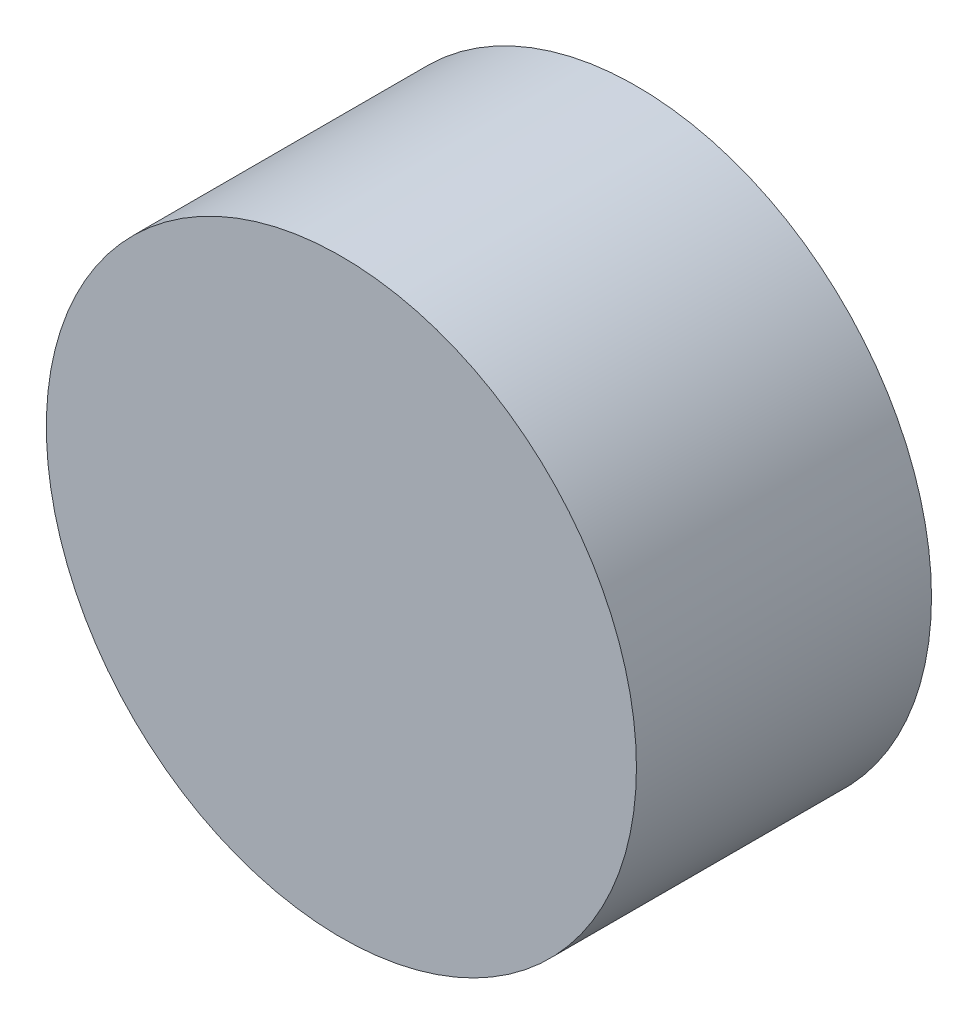
SolidWorks part; units mm, degrees
material "普通碳钢"
ref_plane "Front Plane" through (0, 0, 0) normal (0, 0, 1) x (1, 0, 0)
ref_plane "Top Plane" through (0, 0, 0) normal (0, 1, 0) x (1, 0, 0)
ref_plane "Right Plane" through (0, 0, 0) normal (1, 0, 0) x (0, 0, -1)
sketch "Sketch1" plane through (0, 0, 0) normal (0, 0, 1) x (1, 0, 0)
  circle A0 centre (52.7086, 73.3282) radius 15
  dimension "D1" = 30
extrude "Boss-Extrude1" add sketch "Sketch1" along normal blind 15
